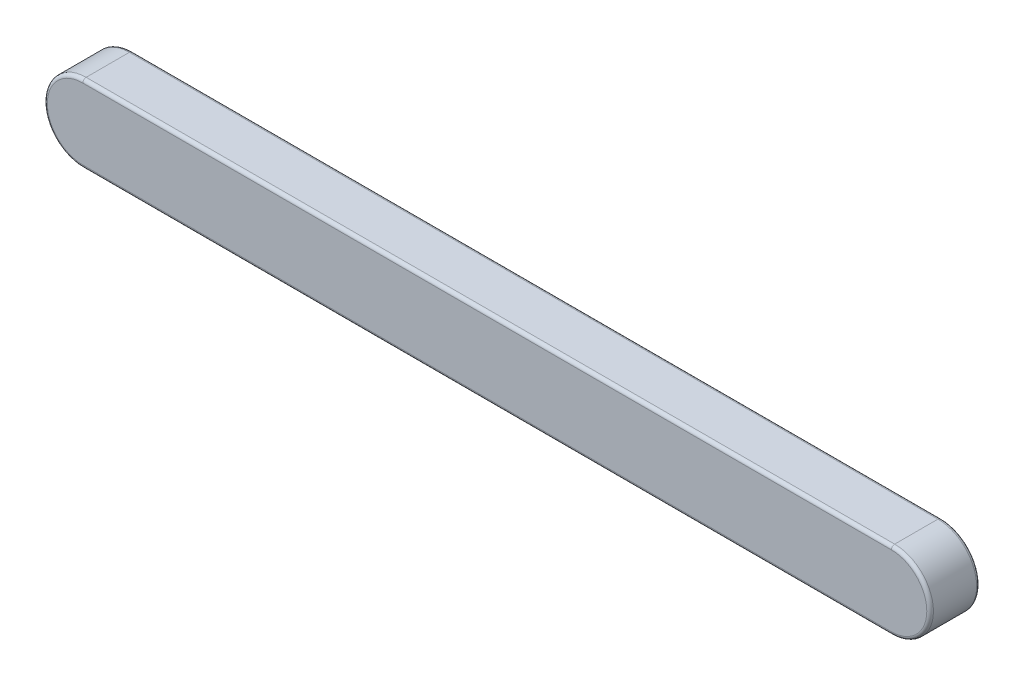
SolidWorks part; units mm, degrees
ref_plane "Plane1" through (0, 0, 0) normal (0, 0, 1) x (1, 0, 0)
ref_plane "Plane2" through (0, 0, 0) normal (0, 1, 0) x (1, 0, 0)
ref_plane "Plane3" through (0, 0, 0) normal (1, 0, 0) x (0, 0, -1)
sketch "Dimension Sketch" plane through (0, 0, 0) normal (0, 0, 1) x (1, 0, 0)
  line L0 (-80, 0) -> (80, 0) construction
  point P3 (-9, 0)
  point P4 (-0.6, 0)
  point P5 (0, 0)
  point P8 (-14, 0)
  point P11 (0, 0)
sketch "Sketch1" plane through (0, 0, 0) normal (0, 0, 1) x (1, 0, 0)
  line L0 (-28.0599, 0) -> (30.562, 0) construction
  line L1 (-73, 7) -> (73, 7)
  line L2 (-73, -7) -> (73, -7)
  line L3 (0, 2.9108) -> (0, -2.1805) construction
  arc A0 (-73, 7) -> (-73, -7) centre (-73, 0) ccw
  arc A1 (73, 7) -> (73, -7) centre (73, 0) cw
extrude "Base-Extrude" add sketch "Sketch1" along normal blind 9
fillet "Fillet1" radius 0.6 8 edges at (80, 0, 9) (0, 7, 9) (-80, 0, 9) (0, 7, 0) (80, 0, 0) (0, -7, 0) (-80, 0, 0) (0, -7, 9)
equation "\"D3@Sketch1\" = \"L@Dimension Sketch\""
equation "\"D1@Sketch1\" = \"b@Dimension Sketch\" / 2"
equation "\"D1@Fillet1\" = \"r@Dimension Sketch\""
equation "\"D1@Base-Extrude\" = \"h@Dimension Sketch\""
